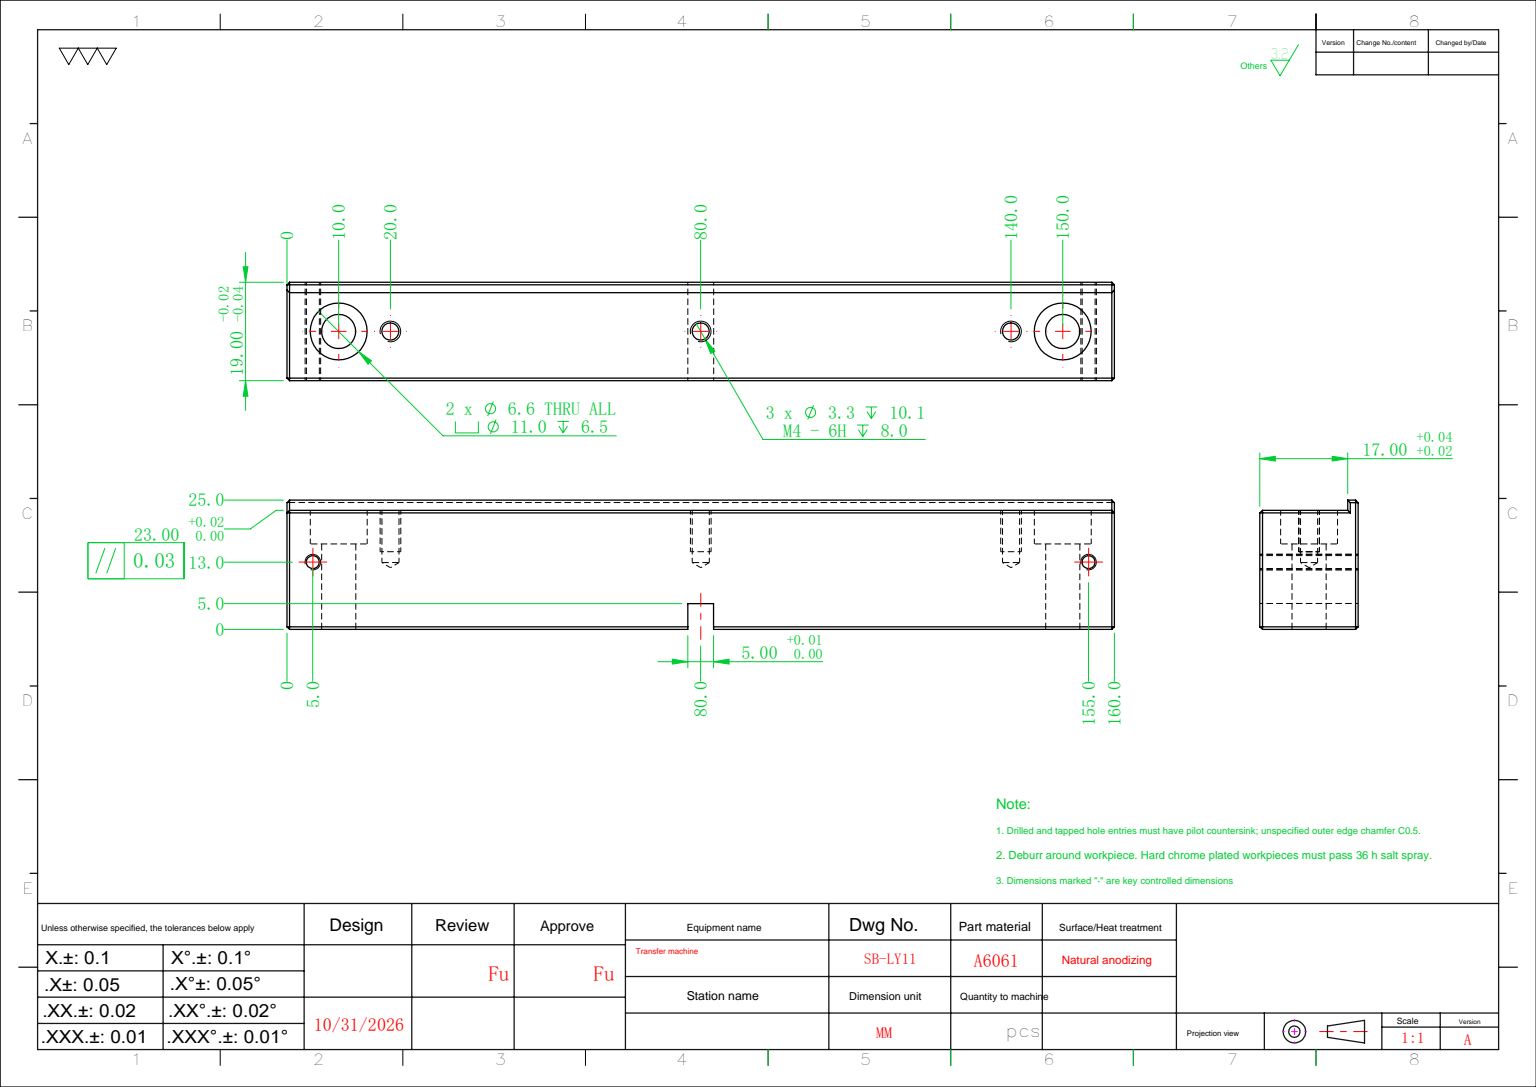
SolidWorks part; units mm, degrees
material "A6061"
ref_plane "前视基准面" through (0, 0, 0) normal (0, 0, 1) x (1, 0, 0)
ref_plane "上视基准面" through (0, 0, 0) normal (0, 1, 0) x (1, 0, 0)
ref_plane "右视基准面" through (0, 0, 0) normal (1, 0, 0) x (0, 0, -1)
sketch "草图1" plane through (0, 0, 0) normal (0, 0, 1) x (1, 0, 0)
  line L1 (-80, -12.5) -> (80, -12.5)
  line L2 (-80, -12.5) -> (-80, 12.5)
  line L3 (-80, 12.5) -> (80, 12.5)
  line L4 (80, -12.5) -> (80, 12.5)
  line L5 (-80, -12.5) -> (80, 12.5) construction
  line L6 (-80, 12.5) -> (80, -12.5) construction
  point P0 (0, 0)
  dimension "D1" = 160
  dimension "D2" = 25
extrude "凸台-拉伸1" add sketch "草图1" along normal blind 19
sketch "草图2" plane through (0, -12.5, 0) normal (0, -1, 0) x (1, 0, 0)
  line L0 (80, 19) -> (80, 0) construction
  line L1 (80, 2) -> (-80, 2)
  line L2 (80, 2) -> (80, 17)
  line L3 (80, 17) -> (-80, 17)
  line L4 (-80, 2) -> (-80, 17)
  line L5 (-80, 19) -> (-80, 0) construction
  line L6 (-80, 9.5) -> (22.243, 9.5) construction
  dimension "D1" = 15
extrude "切除-拉伸1" cut sketch "草图2" against normal blind 2
hole_wizard "M4 螺纹孔1" positions "草图3" profile "草图4" tap size "M4" standard "ISO"
sketch "草图3" plane through (0, -10.5, 0) normal (0, -1, 0) x (-1, 0, 0)
  line L0 (-80, -9.5) -> (80, -9.5) construction
  line L1 (-80, -2) -> (-80, -17) construction
  line L2 (80, -17) -> (80, -2) construction
  point P0 (-60, -9.5)
  point P3 (0, -9.5)
  point P6 (60, -9.5)
  dimension "D1" = 20
  dimension "D2" = 60
  dimension "D3" = 60
sketch "草图4" plane through (60, -10.5, 9.5) normal (1, 0, 0) x (0, 0, -1)
  line L0 (0, 0) -> (0, 11.0914)
  line L1 (0, 11.0914) -> (1.65, 10.1)
  line L2 (1.65, 10.1) -> (1.65, 0)
  line L5 (1.65, 0) -> (0, 0)
  line L10 (0, 11.0914) -> (-1.65, 10.1) construction
  line L11 (0, -6.35) -> (0, 107.95) construction
  dimension "螺纹孔钻头直径" = 3.3
  dimension "螺纹孔钻头深度" = 10.1
  dimension "导头角度" = 118
cosmetic thread "孔螺蚊线1" parameters "D1"=8, "D2"=4
cosmetic thread "孔螺蚊线2" parameters "D1"=8, "D2"=4
cosmetic thread "孔螺蚊线3" parameters "D1"=8, "D2"=4
hole_wizard "M6 六角凹头螺钉的柱形沉头孔1" positions "草图5" profile "草图6" counterbore size "M6" standard "ISO" end condition through all
sketch "草图5" plane through (0, -10.5, 0) normal (0, -1, 0) x (-1, 0, 0)
  line L0 (80, -9.5) -> (-80, -9.5) construction
  line L1 (80, -17) -> (80, -2) construction
  line L2 (-80, -2) -> (-80, -17) construction
  line L4 (0, 0) -> (0, -30.2286) construction
  point P0 (-70, -9.5)
  point P2 (70, -9.5)
  dimension "D1" = 140
sketch "草图6" plane through (70, -10.5, 9.5) normal (1, 0, 0) x (0, 0, -1)
  line L0 (0, 0) -> (0, 23)
  line L1 (0, 23) -> (3.3, 23)
  line L3 (3.3, 23) -> (3.3, 6.5)
  line L4 (3.3, 6.5) -> (5.5, 6.5)
  line L5 (5.5, 6.5) -> (5.5, 0)
  line L7 (5.5, 0) -> (0, 0)
  line L11 (0, -6.35) -> (0, 107.95) construction
  dimension "通孔孔直径" = 6.6
  dimension "通孔孔深度" = 23
  dimension "柱形沉头孔直径" = 11
  dimension "柱形沉头孔深度" = 6.5
sketch "草图7" plane through (0, 0, 19) normal (0, 0, 1) x (1, 0, 0)
  line L0 (80, 12.5) -> (-80, 12.5) construction
  line L1 (-2.5, 12.5) -> (2.5, 12.5)
  line L2 (-2.5, 12.5) -> (-2.5, 7.5)
  line L3 (-2.5, 7.5) -> (2.5, 7.5)
  line L4 (2.5, 12.5) -> (2.5, 7.5)
  line L5 (0, 0) -> (0, 16.0493) construction
  dimension "D1" = 5
  dimension "D2" = 5
extrude "切除-拉伸2" cut sketch "草图7" against normal through all
sketch "草图10" plane through (80, 0, 0) normal (1, 0, 0) x (0, 0, -1)
  line L1 (-17, -10.5) -> (-19, -10.5)
  line L2 (-17, -10.5) -> (-17, -12.5)
  line L3 (-17, -12.5) -> (-19, -12.5)
  line L4 (-19, -10.5) -> (-19, -12.5)
extrude "切除-拉伸3" cut sketch "草图10" against normal through all
chamfer "倒角1" distance 0.5 angle 45 18 edges at (80, -12.5, 1) (80, 1, 19) (41.25, 12.5, 19) (80, 12.5, 9.5) (80, -10.5, 10.5) (80, -11.5, 2) (-80, 0, 0) (-41.25, 12.5, 0) (-80, 12.5, 9.5) (-41.25, 12.5, 19) (-80, 1, 19) (-80, -10.5, 10.5) (-80, -11.5, 2) (-80, -12.5, 1) (0, -12.5, 0) (80, 0, 0) (41.25, 12.5, 0) (0, -10.5, 19)
hole_wizard "M3 螺纹孔1" positions "草图8" profile "草图9" tap size "M3" standard "ISO" end condition through all
sketch "草图8" plane through (0, 0, 19) normal (0, 0, 1) x (1, 0, 0)
  line L0 (0, 0) -> (0, -29.9927) construction
  line L2 (2.5, 12.5) -> (79.5, 12.5) construction
  point P0 (75, -0.5)
  point P2 (-75, -0.5)
  dimension "D1" = 150
  dimension "D2" = 13
sketch "草图9" plane through (75, -0.5, 19) normal (1, 0, 0) x (0, -1, 0)
  line L0 (0, 0) -> (0, 19)
  line L1 (0, 19) -> (1.25, 19)
  line L2 (1.25, 19) -> (1.25, 0)
  line L5 (1.25, 0) -> (0, 0)
  line L11 (0, -6.35) -> (0, 107.95) construction
  dimension "通孔螺纹孔钻头直径" = 2.5
  dimension "通孔螺纹孔钻头深度" = 19
cosmetic thread "孔螺蚊线4" parameters "D2"=3
cosmetic thread "孔螺蚊线5" parameters "D2"=3
